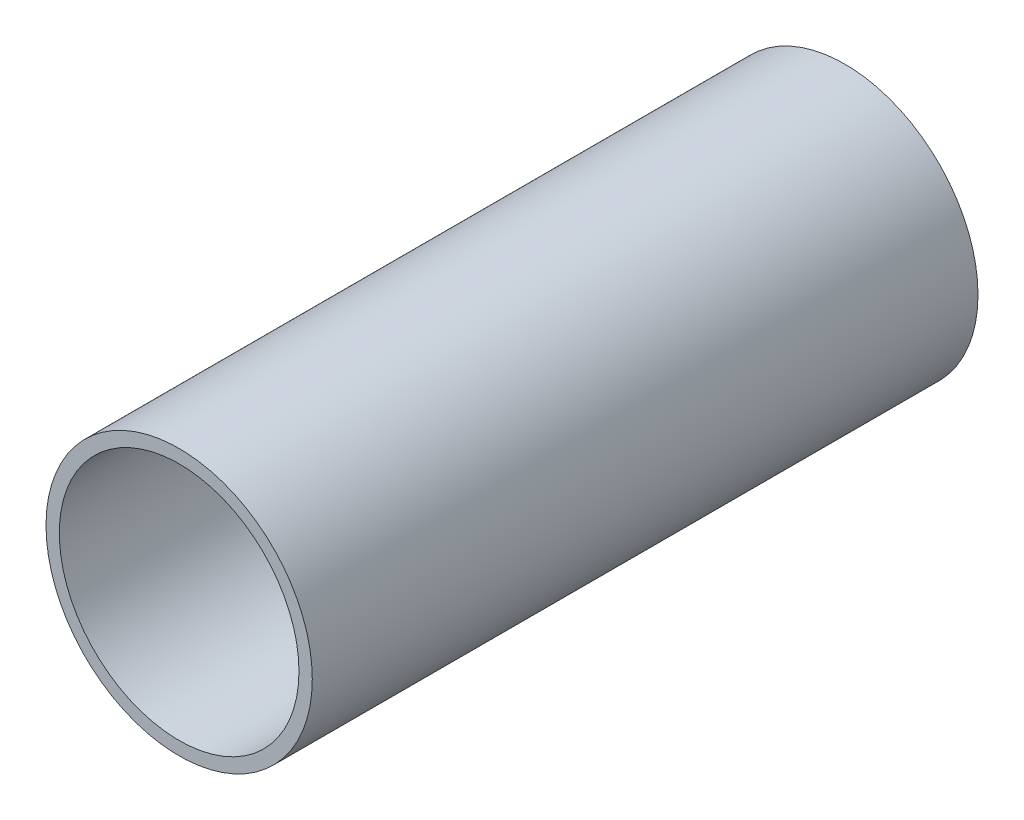
from build123d import *

# Parameters (mm, degrees)
SKETCH1_R           = 30
SKETCH1_R_2         = 27
BOSS_EXTRUDE1_DEPTH = 150


with BuildPart() as part:
    # Sketch1 → Boss-Extrude1 (new body)
    with BuildSketch(Plane.XY):
        Circle(SKETCH1_R)
        Circle(SKETCH1_R_2, mode=Mode.SUBTRACT)
    extrude(amount=BOSS_EXTRUDE1_DEPTH)


solid = part.part
